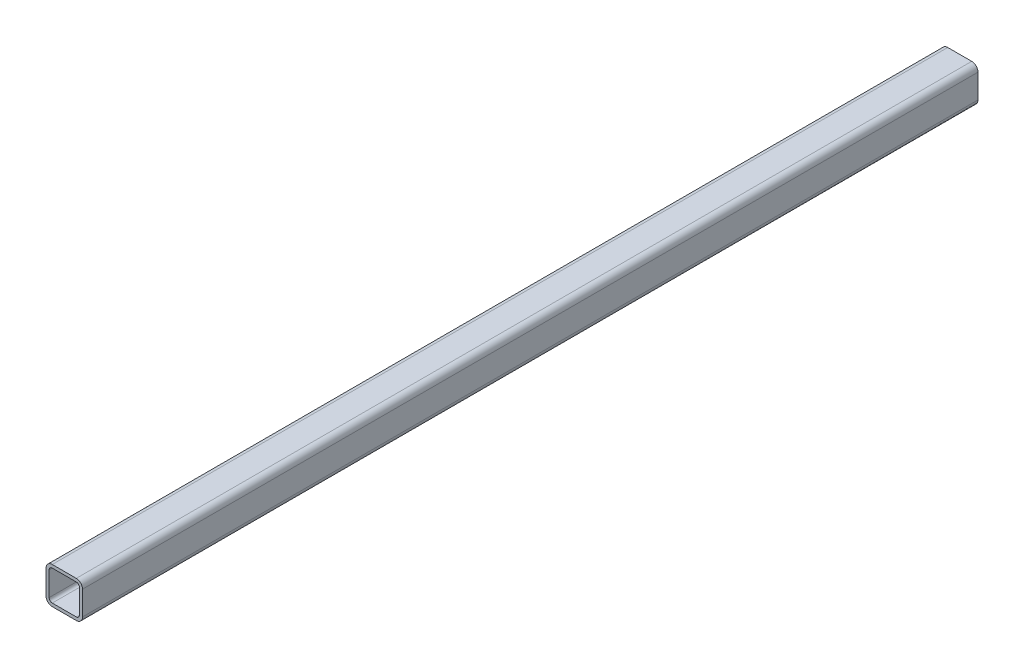
SolidWorks part; units mm, degrees
material "方管70×6/不锈钢304"
ref_plane "Front Plane" through (0, 0, 0) normal (0, 0, 1) x (1, 0, 0)
ref_plane "Top Plane" through (0, 0, 0) normal (0, 1, 0) x (1, 0, 0)
ref_plane "Right Plane" through (0, 0, 0) normal (1, 0, 0) x (0, 0, -1)
sketch "Sketch1" plane through (0, 0, 0) normal (0, 0, 1) x (1, 0, 0)
  line L1 (12, 0) -> (58, 0)
  line L2 (0, 12) -> (0, 58)
  line L3 (12, 70) -> (58, 70)
  line L4 (70, 12) -> (70, 58)
  line L5 (12, 6) -> (58, 6)
  line L6 (6, 12) -> (6, 58)
  line L7 (12, 64) -> (58, 64)
  line L8 (64, 12) -> (64, 58)
  arc A0 (12, 6) -> (6, 12) centre (12, 12) cw
  arc A1 (58, 6) -> (64, 12) centre (58, 12) ccw
  arc A2 (58, 64) -> (64, 58) centre (58, 58) cw
  arc A3 (6, 58) -> (12, 64) centre (12, 58) cw
  arc A4 (12, 0) -> (0, 12) centre (12, 12) cw
  arc A5 (58, 0) -> (70, 12) centre (58, 12) ccw
  arc A6 (58, 70) -> (70, 58) centre (58, 58) cw
  arc A7 (0, 58) -> (12, 70) centre (12, 58) cw
  point P19 (0, 0)
  point P22 (70, 0)
  point P27 (0, 70)
  dimension "D7" = 6
  dimension "D8" = 12
  dimension "D1" = 70
  dimension "D2" = 70
  dimension "D3" = 6
  dimension "D4" = 6
  dimension "D5" = 6
  dimension "D6" = 6
extrude "Boss-Extrude1" add sketch "Sketch1" along normal blind 1716
